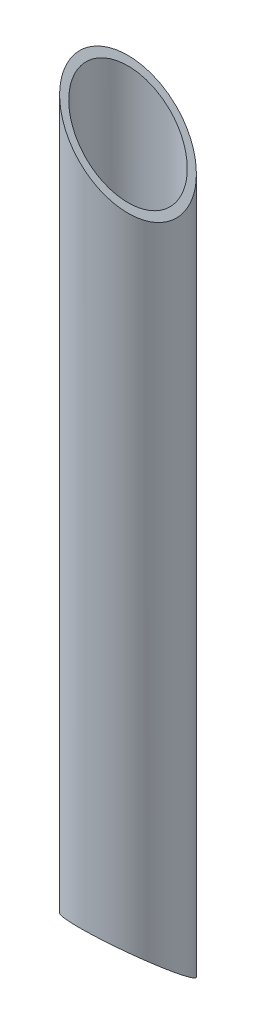
SolidWorks part; units mm, degrees
material "Q235"
ref_plane "Front Plane" through (0, 0, 0) normal (0, 0, 1) x (1, 0, 0)
ref_plane "Top Plane" through (0, 0, 0) normal (0, 1, 0) x (1, 0, 0)
ref_plane "Right Plane" through (0, 0, 0) normal (1, 0, 0) x (0, 0, -1)
sketch "Sketch1" plane through (0, 0, 0) normal (0, 1, 0) x (1, 0, 0)
  circle A0 centre (0, 0) radius 30
  circle A1 centre (0, 0) radius 26
  dimension "D1" = 4
  dimension "D2" = 60
extrude "Boss-Extrude1" add sketch "Sketch1" along normal blind 490
sketch "Sketch2" plane through (0, 0, 0) normal (0, 0, 1) x (1, 0, 0)
  line L0 (-30, 490) -> (243.2123, 216.7877)
  line L1 (30, 490) -> (-30, 490) construction
  dimension "D1" = 45
extrude "Cut-Extrude1" cut sketch "Sketch2" against normal through all both and the other way through all
sketch "Sketch3" plane through (0, 0, 0) normal (1, 0, 0) x (0, 0, -1)
  line L0 (30, 0) -> (-69.8826, 80.8834)
  line L2 (-30, 0) -> (30, 0) construction
  dimension "D1" = 39
extrude "Cut-Extrude2" cut sketch "Sketch3" against normal through all both and the other way through all
